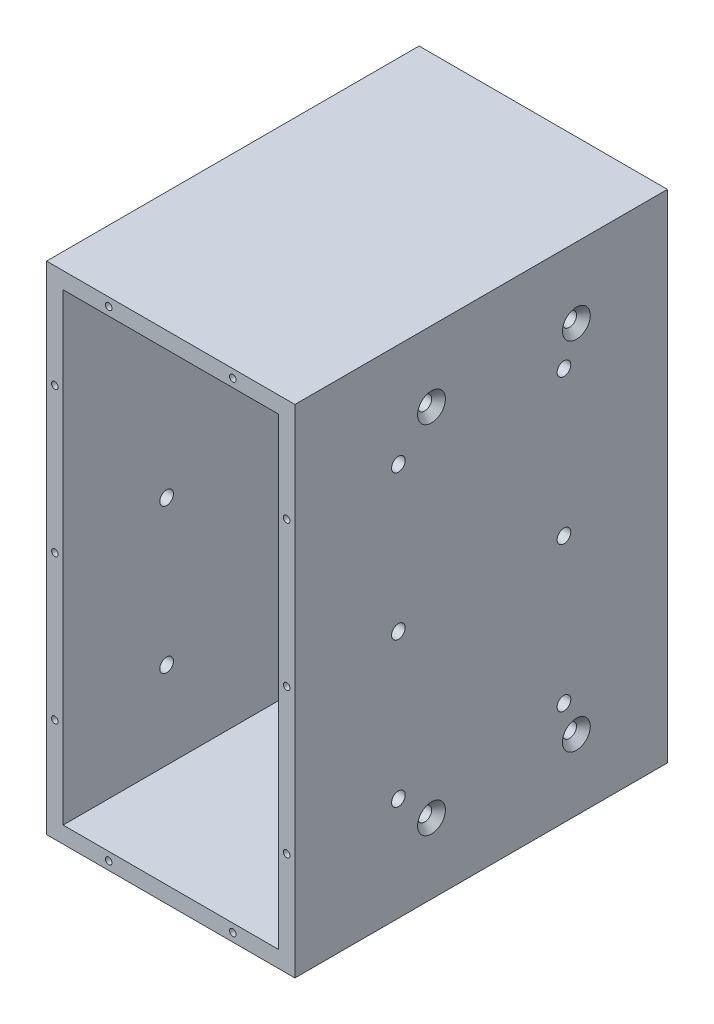
SolidWorks part; units mm, degrees
material "6061Al"
ref_plane "前视基准面" through (0, 0, 0) normal (0, 0, 1) x (1, 0, 0)
ref_plane "上视基准面" through (0, 0, 0) normal (0, 1, 0) x (1, 0, 0)
ref_plane "右视基准面" through (0, 0, 0) normal (1, 0, 0) x (0, 0, -1)
sketch "草图1" plane through (0, 0, 0) normal (0, 0, 1) x (1, 0, 0)
  line L1 (-30, -60) -> (30, -60)
  line L2 (-30, -60) -> (-30, 60)
  line L3 (-30, 60) -> (30, 60)
  line L4 (30, -60) -> (30, 60)
  line L5 (-30, -60) -> (30, 60) construction
  line L6 (-30, 60) -> (30, -60) construction
  point P0 (0, 0)
  dimension "D1" = 120
  dimension "D2" = 60
extrude "凸台-拉伸1" add sketch "草图1" along normal mid plane 90
shell "抽壳1" thickness 4
hole_wizard "M2 螺纹孔1" positions "草图7" profile "草图8" tap size "M2" standard "ISO"
sketch "草图7" plane through (0, 0, 45) normal (0, 0, 1) x (1, 0, 0)
  line L13 (28, -58) -> (28, 58)
  line L14 (28, 58) -> (-28, 58)
  line L15 (-28, 58) -> (-28, -58)
  line L16 (-28, -58) -> (28, -58)
  line L17 (28, -58) -> (28, 58)
  line L18 (28, 58) -> (-28, 58)
  line L19 (-28, 58) -> (-28, -58)
  line L20 (-28, -58) -> (28, -58)
  line L21 (0, 0) -> (0, 71.2849) construction
  line L23 (0, 0) -> (54.0936, 0) construction
  line L41 (28, -58) -> (-28, -58)
  point P74 (-28, 0)
  point P82 (28, 0)
  point P99 (-15, 58)
  point P101 (15, 58)
  point P103 (-28, 35)
  point P105 (28, 35)
  point P119 (28, -35)
  point P120 (-28, -35)
  point P155 (15, -58)
  point P156 (-15, -58)
  dimension "D1" = 2
  dimension "D2" = 70
  dimension "D3" = 30
sketch "草图8" plane through (-15, -58, 45) normal (1, 0, 0) x (0, -1, 0)
  line L0 (0, 0) -> (0, 5.6807)
  line L1 (0, 5.6807) -> (0.8, 5.2)
  line L2 (0.8, 5.2) -> (0.8, 0)
  line L5 (0.8, 0) -> (0, 0)
  line L10 (0, 5.6807) -> (-0.8, 5.2) construction
  line L11 (0, -6.35) -> (0, 107.95) construction
  dimension "螺纹孔钻头直径" = 1.6
  dimension "螺纹孔钻头深度" = 5.2
  dimension "导头角度" = 118
cosmetic thread "孔螺蚊线1" parameters "D1"=4, "D2"=2
cosmetic thread "孔螺蚊线2" parameters "D1"=4, "D2"=2
cosmetic thread "孔螺蚊线3" parameters "D1"=4, "D2"=2
cosmetic thread "孔螺蚊线4" parameters "D1"=4, "D2"=2
cosmetic thread "孔螺蚊线5" parameters "D1"=4, "D2"=2
cosmetic thread "孔螺蚊线6" parameters "D1"=4, "D2"=2
cosmetic thread "孔螺蚊线7" parameters "D1"=4, "D2"=2
cosmetic thread "孔螺蚊线8" parameters "D1"=4, "D2"=2
cosmetic thread "孔螺蚊线17" parameters "D1"=4, "D2"=2
cosmetic thread "孔螺蚊线19" parameters "D1"=4, "D2"=2
hole_wizard "M2 螺纹孔2" positions "草图9" profile "草图10" tap size "M2" standard "ISO"
sketch "草图9" plane through (0, 0, -45) normal (0, 0, -1) x (-1, 0, 0)
  point P9 (28, 0)
  point P21 (-28, 0)
  point P26 (-15, 58)
  point P29 (15, 58)
  point P32 (28, 35)
  point P35 (-28, 35)
  point P38 (-28, -35)
  point P44 (28, -35)
  point P48 (-15, -58)
  point P51 (15, -58)
cosmetic thread "孔螺蚊线9" parameters "D1"=4, "D2"=2
cosmetic thread "孔螺蚊线10" parameters "D1"=4, "D2"=2
cosmetic thread "孔螺蚊线11" parameters "D1"=4, "D2"=2
cosmetic thread "孔螺蚊线12" parameters "D1"=4, "D2"=2
cosmetic thread "孔螺蚊线13" parameters "D1"=4, "D2"=2
cosmetic thread "孔螺蚊线14" parameters "D1"=4, "D2"=2
cosmetic thread "孔螺蚊线15" parameters "D1"=4, "D2"=2
cosmetic thread "孔螺蚊线16" parameters "D1"=4, "D2"=2
sketch "草图10" plane through (-28, 0, -45) normal (1, 0, 0) x (0, 1, 0)
  line L0 (0, 0) -> (0, 5.6807)
  line L1 (0, 5.6807) -> (0.8, 5.2)
  line L2 (0.8, 5.2) -> (0.8, 0)
  line L5 (0.8, 0) -> (0, 0)
  line L10 (0, 5.6807) -> (-0.8, 5.2) construction
  line L11 (0, -6.35) -> (0, 107.95) construction
  dimension "螺纹孔钻头直径" = 1.6
  dimension "螺纹孔钻头深度" = 5.2
  dimension "导头角度" = 118
cosmetic thread "孔螺蚊线18" parameters "D1"=4, "D2"=2
cosmetic thread "孔螺蚊线20" parameters "D1"=4, "D2"=2
hole_wizard "M3 六角凹锥坑螺钉的锥形沉头孔1" positions "草图11" profile "草图12" countersink size "M3" standard "ISO"
sketch "草图11" plane through (30, 0, 0) normal (1, 0, 0) x (0, 0, -1)
  point P0 (-12, 43)
  point P3 (23, 43)
  point P6 (-12, -43)
  point P9 (23, -43)
sketch "草图12" plane through (30, 43, 12) normal (0, 1, 0) x (0, 0, -1)
  line L0 (0, 0) -> (0, 4)
  line L1 (0, 4) -> (1.7, 4)
  line L2 (1.7, 4) -> (1.7, 1.66)
  line L3 (1.7, 1.66) -> (3.36, 0)
  line L5 (3.36, 0) -> (0, 0)
  line L6 (-1.7, 1.66) -> (-3.36, 0) construction
  line L11 (0, -6.35) -> (0, 107.95) construction
  dimension "通孔孔直径" = 3.4
  dimension "通孔孔深度" = 4
  dimension "近端锥形沉头孔直径" = 6.72
  dimension "近端锥形沉头孔角度" = 90
hole_wizard "M4 螺纹孔1" positions "草图13" profile "草图14" tap size "M4" standard "ISO" end condition through all
sketch "草图13" plane through (30, 0, 0) normal (1, 0, 0) x (0, 0, -1)
  line L1 (-20, -35) -> (20, -35)
  line L2 (-20, -35) -> (-20, 35)
  line L3 (-20, 35) -> (20, 35)
  line L4 (20, -35) -> (20, 35)
  line L5 (-20, -35) -> (20, 35) construction
  line L6 (-20, 35) -> (20, -35) construction
  point P2 (20, 35)
  point P5 (-20, -35)
  point P6 (-20, 35)
  point P7 (20, -35)
  point P84 (-20, 0)
  point P86 (20, 0)
  dimension "D1" = 40
  dimension "D2" = 70
sketch "草图14" plane through (30, 35, -20) normal (0, 1, 0) x (0, 0, -1)
  line L0 (0, 0) -> (0, 60)
  line L1 (0, 60) -> (1.65, 60)
  line L2 (1.65, 60) -> (1.65, 0)
  line L5 (1.65, 0) -> (0, 0)
  line L11 (0, -6.35) -> (0, 107.95) construction
  dimension "通孔螺纹孔钻头直径" = 3.3
  dimension "通孔螺纹孔钻头深度" = 60
cosmetic thread "孔螺蚊线21" parameters "D2"=4
cosmetic thread "孔螺蚊线22" parameters "D2"=4
cosmetic thread "孔螺蚊线23" parameters "D2"=4
cosmetic thread "孔螺蚊线24" parameters "D2"=4
cosmetic thread "孔螺蚊线25" parameters "D2"=4
cosmetic thread "孔螺蚊线26" parameters "D2"=4
